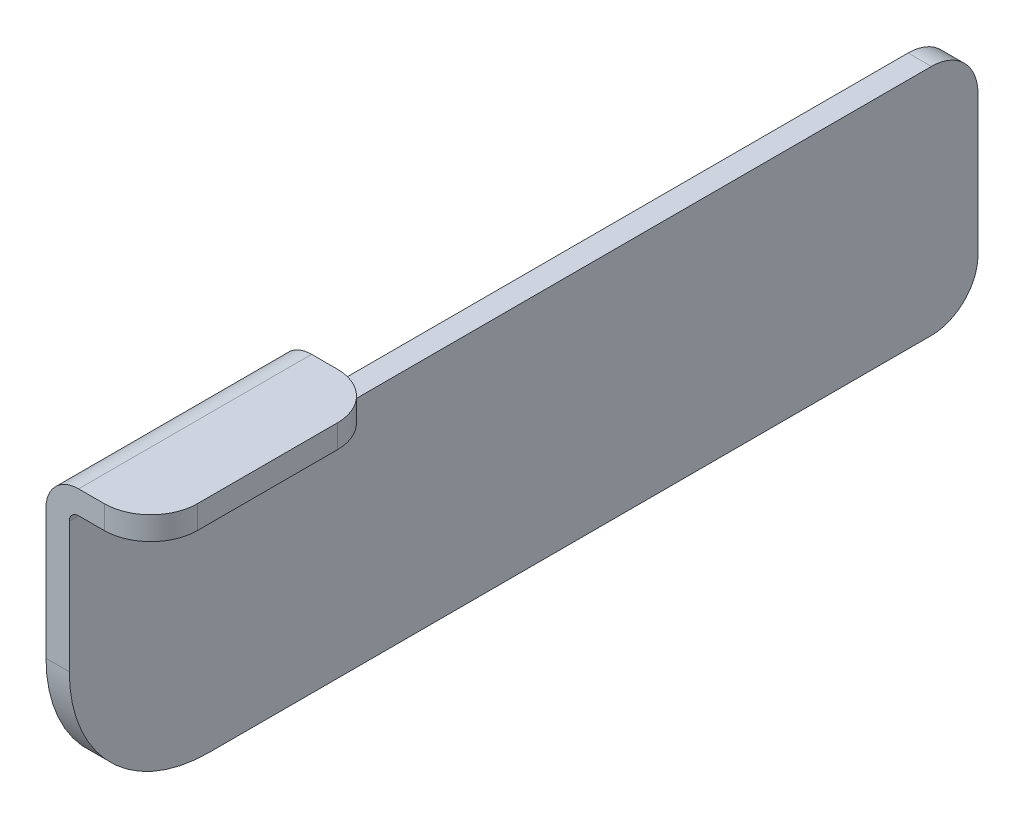
from build123d import *

# Parameters (mm, degrees)
EXTRUDE_THIN1_DEPTH = 100
SKETCH2_W           = 10
SKETCH2_H           = 100
BOSS_EXTRUDE1_DEPTH = 290
FILLET1_R           = 60
FILLET2_R           = 20
FILLET3_R           = 10
SKETCH3_R           = 6
CUT_EXTRUDE1_DEPTH  = 6
LPATTERN1_COUNT     = 2
LPATTERN1_PITCH     = 70
SKETCH4_R           = 5.5
CUT_EXTRUDE2_DEPTH  = 6
LPATTERN2_COUNT     = 2
LPATTERN2_PITCH     = 60


with BuildPart() as part:
    # Sketch1 → Extrude-Thin1 (new body)
    with BuildSketch(Plane.XY):
        with BuildLine():
            Line((0, -130), (0, -14))
            ThreePointArc((0, -14), (4.100505063, -4.100505063), (14, 0))
            Line((14, 0), (45, 0))
            Line((45, 0), (45, -10))
            Line((45, -10), (14, -10))
            ThreePointArc((14, -10), (11.171572875, -11.171572875), (10, -14))
            Line((10, -14), (10, -130))
            Line((10, -130), (0, -130))
        make_face()
    extrude(amount=EXTRUDE_THIN1_DEPTH)

    # Sketch2 → Boss-Extrude1 (add)
    with BuildSketch(Plane(origin=(0, 0, 0), x_dir=(-1, 0, 0), z_dir=(0, 0, -1))):
        with Locations((-5, -80)):
            Rectangle(SKETCH2_W, SKETCH2_H)
    extrude(amount=BOSS_EXTRUDE1_DEPTH)

    # Fillet1
    fillet1_edges = [part.edges().sort_by_distance(p)[0] for p in [
        (5, -130, 100),
    ]]
    fillet(fillet1_edges, radius=FILLET1_R)

    # Fillet2
    fillet2_edges = [part.edges().sort_by_distance(p)[0] for p in [
        (5, -30, -290),
        (5, -130, -290),
        (45, -5, 0),
        (45, -5, 100),
    ]]
    fillet(fillet2_edges, radius=FILLET2_R)

    # Fillet3
    fillet3_edges = [part.edges().sort_by_distance(p)[0] for p in [
        (5, -30, 0),
    ]]
    fillet(fillet3_edges, radius=FILLET3_R)

    # Sketch3 → Cut-Extrude1 (cut)
    with BuildSketch(Plane.XZ.offset(10)):
        with Locations(Location((30, 85, 0), (0, 0, 270))):
            Circle(SKETCH3_R)
    cut_extrude1 = extrude(amount=-CUT_EXTRUDE1_DEPTH, mode=Mode.SUBTRACT)

    # LPattern1: Cut-Extrude1 ×2
    with Locations(*[(0, 0, -i * LPATTERN1_PITCH) for i in range(1, LPATTERN1_COUNT)]):
        add(cut_extrude1, mode=Mode.SUBTRACT)

    # Sketch4 → Cut-Extrude2 (cut)
    with BuildSketch(Plane.ZY):
        with Locations(Location((-275, -50, 0), (0, 0, 270))):
            Circle(SKETCH4_R)
    cut_extrude2 = extrude(amount=-CUT_EXTRUDE2_DEPTH, mode=Mode.SUBTRACT)

    # LPattern2: Cut-Extrude2 ×2
    with Locations(*[(0, -i * LPATTERN2_PITCH, 0) for i in range(1, LPATTERN2_COUNT)]):
        add(cut_extrude2, mode=Mode.SUBTRACT)


solid = part.part
